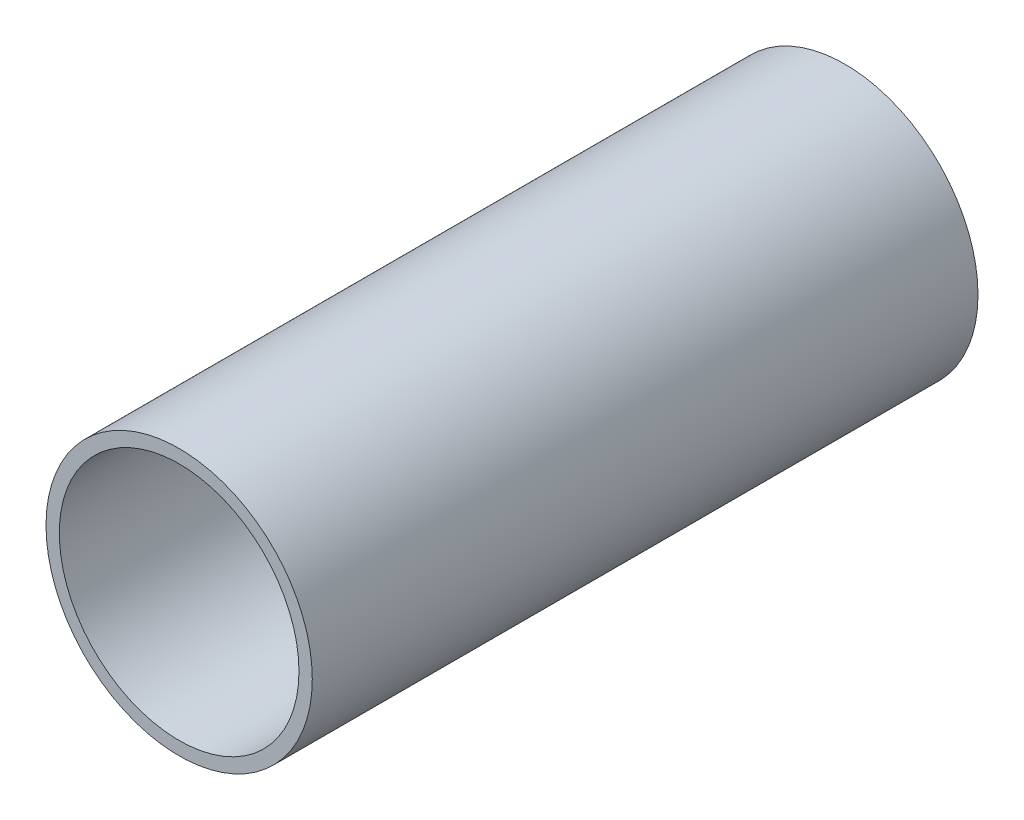
SolidWorks part; units mm, degrees
material "Q235B"
ref_plane "Plane1" through (0, 0, 0) normal (0, 0, 1) x (1, 0, 0)
ref_plane "Plane2" through (0, 0, 0) normal (0, 1, 0) x (1, 0, 0)
ref_plane "Plane3" through (0, 0, 0) normal (1, 0, 0) x (0, 0, -1)
sketch "Sketch1" plane through (0, 0, 0) normal (0, 0, 1) x (1, 0, 0)
  circle A0 centre (0, 0) radius 27
  circle A1 centre (0, 0) radius 30
extrude "Boss-Extrude1" add sketch "Sketch1" along normal blind 150 contours A1 | A0
